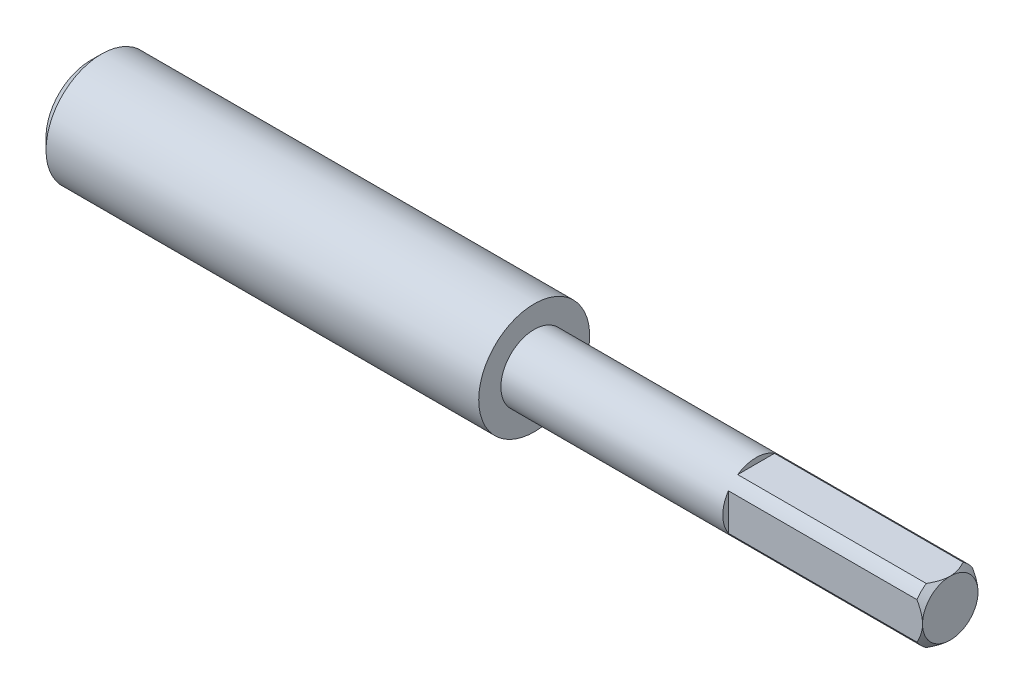
from build123d import *

# Parameters (mm, degrees)
CHAMFER1_SIZE       = 1
CHAMFER2_SIZE       = 2
SKETCH2_OUTSIDE_W   = 53.512
SKETCH2_OUTSIDE_H   = 53.512
SKETCH2_OUTSIDE_W_2 = 10
SKETCH2_OUTSIDE_H_2 = 10
CUT_EXTRUDE1_DEPTH  = 35


with BuildPart() as part:
    # Sketch1 → Revolve1 (revolve)
    with BuildSketch(Plane.XY, mode=Mode.PRIVATE) as revolve1_sk:
        Polygon((0, 0), (0, 10), (80, 10), (80, 6), (155, 6), (155, 0), align=None)
    revolve(revolve1_sk.sketch.rotate(Axis((0, 0, 0), (1, 0, 0)), 90), axis=Axis((0, 0, 0), (1, 0, 0)))

    # Chamfer1
    chamfer1_edges = [part.edges().sort_by_distance(p)[0] for p in [
        (155, 0, -6),
    ]]
    chamfer(chamfer1_edges, length=CHAMFER1_SIZE)

    # Chamfer2
    chamfer2_edges = [part.edges().sort_by_distance(p)[0] for p in [
        (0, 0, -10),
    ]]
    chamfer(chamfer2_edges, length=CHAMFER2_SIZE)

    # Sketch2 outside → Cut-Extrude1 (cut)
    with BuildSketch(Plane(origin=(155, 0, 0), x_dir=(0, 0, -1), z_dir=(1, 0, 0))):
        Rectangle(SKETCH2_OUTSIDE_W, SKETCH2_OUTSIDE_H)
        Rectangle(SKETCH2_OUTSIDE_W_2, SKETCH2_OUTSIDE_H_2, mode=Mode.SUBTRACT)
    extrude(amount=-CUT_EXTRUDE1_DEPTH, mode=Mode.SUBTRACT)


solid = part.part
